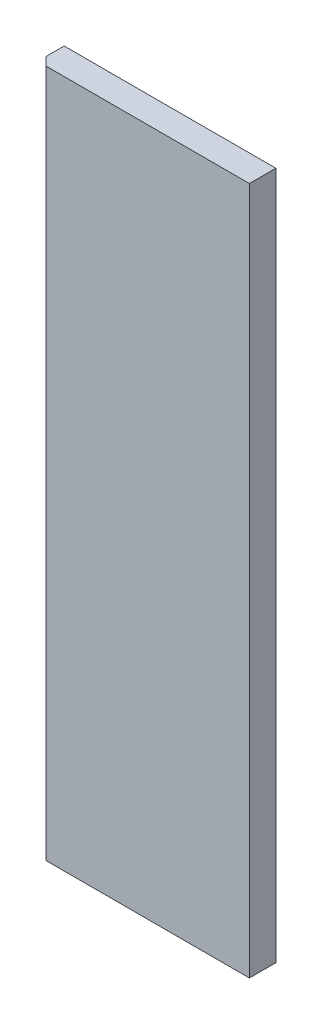
SolidWorks part; units mm, degrees
ref_plane "Front Plane" through (0, 0, 0) normal (0, 0, 1) x (1, 0, 0)
ref_plane "Top Plane" through (0, 0, 0) normal (0, 1, 0) x (1, 0, 0)
ref_plane "Right Plane" through (0, 0, 0) normal (1, 0, 0) x (0, 0, -1)
sketch "Sketch1" plane through (0, 0, 0) normal (0, 0, 1) x (1, 0, 0)
  line L1 (0, 0) -> (200, 0)
  line L2 (0, 0) -> (0, 650)
  line L3 (0, 650) -> (200, 650)
  line L4 (200, 0) -> (200, 650)
  dimension "D1" = 200
  dimension "D2" = 650
extrude "Boss-Extrude1" add sketch "Sketch1" along normal blind 25
chamfer "Chamfer1" distance 8 angle 45 1 edges at (0, 325, 25)
